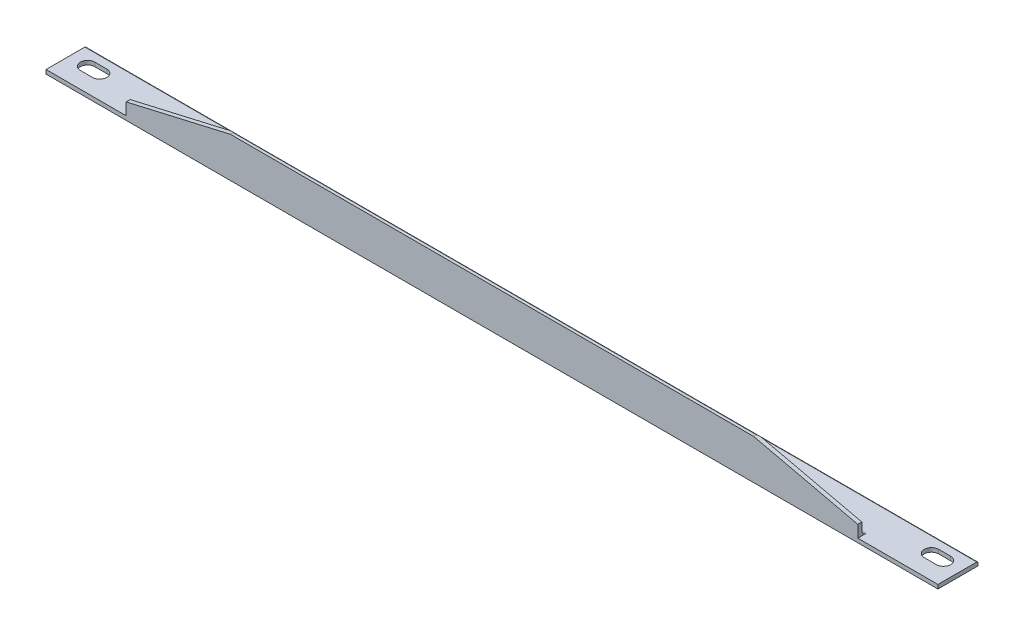
SolidWorks part; units mm, degrees
material "Plain carbon steel"
ref_plane "Front Plane" through (0, 0, 0) normal (0, 0, 1) x (1, 0, 0)
ref_plane "Top Plane" through (0, 0, 0) normal (0, 1, 0) x (1, 0, 0)
ref_plane "Right Plane" through (0, 0, 0) normal (1, 0, 0) x (0, 0, -1)
sketch "Sketch1" plane through (0, 0, 0) normal (0, 0, 1) x (1, 0, 0)
  line L0 (-556.5, 0) -> (556.5, 0)
  dimension "D1" = 1113
other "Hot-rolled equal-leg angle steel (gb t9787-1988) 50×5(1)"
ref_plane "Plane1" through (-556.5, 0, 0) normal (1, 0, 0) x (0, 1, 0)
sketch "Sketch11" plane through (-556.5, 0, 0) normal (1, 0, 0) x (0, 1, 0)
  line L0 (50, 0) -> (0, 0)
  line L1 (0, 0) -> (0, -50)
  line L2 (48.3333, -5) -> (10.5, -5)
  line L3 (5, -10.5) -> (5, -48.3333)
  line L4 (50, 0) -> (50, -3.3333)
  line L5 (0, -50) -> (3.3333, -50)
  arc A0 (50, -3.3333) -> (48.3333, -5) centre (48.3333, -3.3333) cw
  arc A1 (3.3333, -50) -> (5, -48.3333) centre (3.3333, -48.3333) ccw
  arc A2 (10.5, -5) -> (5, -10.5) centre (10.5, -10.5) ccw
  point P2 (25, 0)
  point P13 (0, -25)
  point P15 (0, 0)
  dimension "r1" = 1.6667
  dimension "r" = 5.5
  dimension "b" = 50
  dimension "d" = 5
sketch "Sketch13" plane through (0, 5, 0) normal (0, 1, 0) x (1, 0, 0)
  line L0 (-556.5, 29.4167) -> (556.5, 29.4167) construction
  line L1 (-556.5, 48.3333) -> (-556.5, 10.5) construction
  line L2 (556.5, 48.3333) -> (556.5, 10.5) construction
  line L3 (0, 0) -> (0, 213.456) construction
  line L4 (-534, 29.4167) -> (-519, 29.4167) construction
  line L5 (-534, 38.4167) -> (-519, 38.4167)
  line L6 (-534, 20.4167) -> (-519, 20.4167)
  line L7 (534, 29.4167) -> (519, 29.4167) construction
  line L8 (534, 20.4167) -> (519, 20.4167)
  line L9 (534, 38.4167) -> (519, 38.4167)
  circle A0 centre (526.5, 29.4167) radius 9 construction
  circle A1 centre (-526.5, 29.4167) radius 9 construction
  arc A2 (-534, 38.4167) -> (-534, 20.4167) centre (-534, 29.4167) ccw
  arc A3 (-519, 20.4167) -> (-519, 38.4167) centre (-519, 29.4167) ccw
  arc A4 (534, 20.4167) -> (534, 38.4167) centre (534, 29.4167) ccw
  arc A5 (519, 38.4167) -> (519, 20.4167) centre (519, 29.4167) ccw
  point P12 (-526.5, 29.4167)
  point P22 (526.5, 29.4167)
  dimension "D1" = 18
  dimension "D2" = 30
  dimension "D3" = 18
  dimension "D4" = 30
  dimension "D5" = 15
  dimension "D6" = 15
extrude "Cut-Extrude1" cut sketch "Sketch13" against normal up to next
sketch "Sketch16" plane through (0, 5, 0) normal (0, 1, 0) x (1, 0, 0)
  line L0 (-556.5, 0) -> (556.5, 0) construction
  line L1 (556.5, 10.5) -> (456.5, 10.5)
  line L2 (556.5, 10.5) -> (556.5, 0)
  line L3 (556.5, 0) -> (456.5, 0)
  line L4 (456.5, 10.5) -> (456.5, 0)
  line L6 (-556.5, 10.5) -> (-456.5, 10.5)
  line L7 (-556.5, 10.5) -> (-556.5, 0)
  line L8 (-556.5, 0) -> (-456.5, 0)
  line L9 (-456.5, 10.5) -> (-456.5, 0)
  dimension "D1" = 100
extrude "Cut-Extrude2" cut sketch "Sketch16" along normal up to next
sketch "Sketch17" plane through (0, 0, -5) normal (0, 0, -1) x (-1, 0, 0)
  line L0 (326.5, 50) -> (456.5, 50)
  line L1 (-456.5, 50) -> (456.5, 50) construction
  line L2 (456.5, 50) -> (456.5, 20)
  line L3 (456.5, 10.5) -> (456.5, 48.3333) construction
  line L4 (456.5, 20) -> (326.5, 50)
  line L5 (0, 0) -> (0, 191.5438) construction
  line L6 (-456.5, 20) -> (-326.5, 50)
  line L7 (-456.5, 50) -> (-456.5, 20)
  line L8 (-326.5, 50) -> (-456.5, 50)
  dimension "D1" = 130
  dimension "D2" = 30
extrude "Cut-Extrude3" cut sketch "Sketch17" against normal through all both and the other way through all
